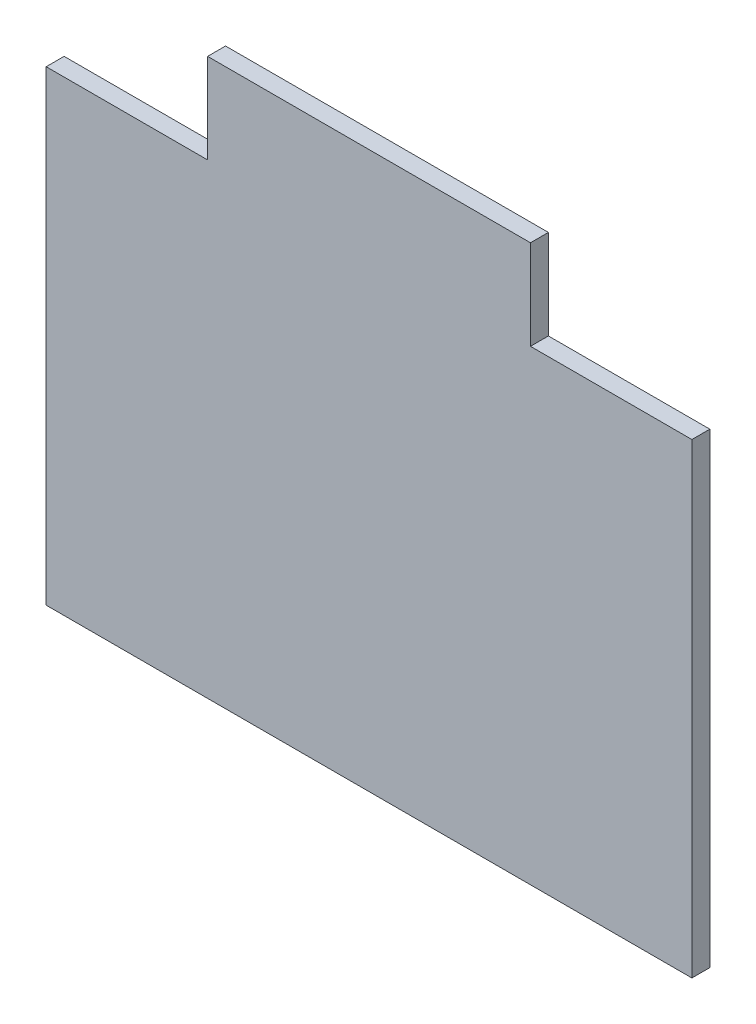
from build123d import *

# Parameters (mm, degrees)
SKETCH_1_W      = 180
SKETCH_1_H      = 130
EXTRUDE_1_DEPTH = 5
SKETCH_2_W      = 90
SKETCH_2_H      = 5
EXTRUDE_2_DEPTH = 25


with BuildPart() as part:
    # 草图1 → 凸台-拉伸1 (new body)
    with BuildSketch(Plane.XY):
        with Locations((90, -65)):
            Rectangle(SKETCH_1_W, SKETCH_1_H)
    extrude(amount=EXTRUDE_1_DEPTH)

    # 草图2 → 凸台-拉伸2 (add)
    with BuildSketch(Plane(origin=(0, 0, 0), x_dir=(1, 0, 0), z_dir=(0, 1, 0))):
        with Locations((90, -2.5)):
            Rectangle(SKETCH_2_W, SKETCH_2_H)
    extrude(amount=EXTRUDE_2_DEPTH)


solid = part.part
